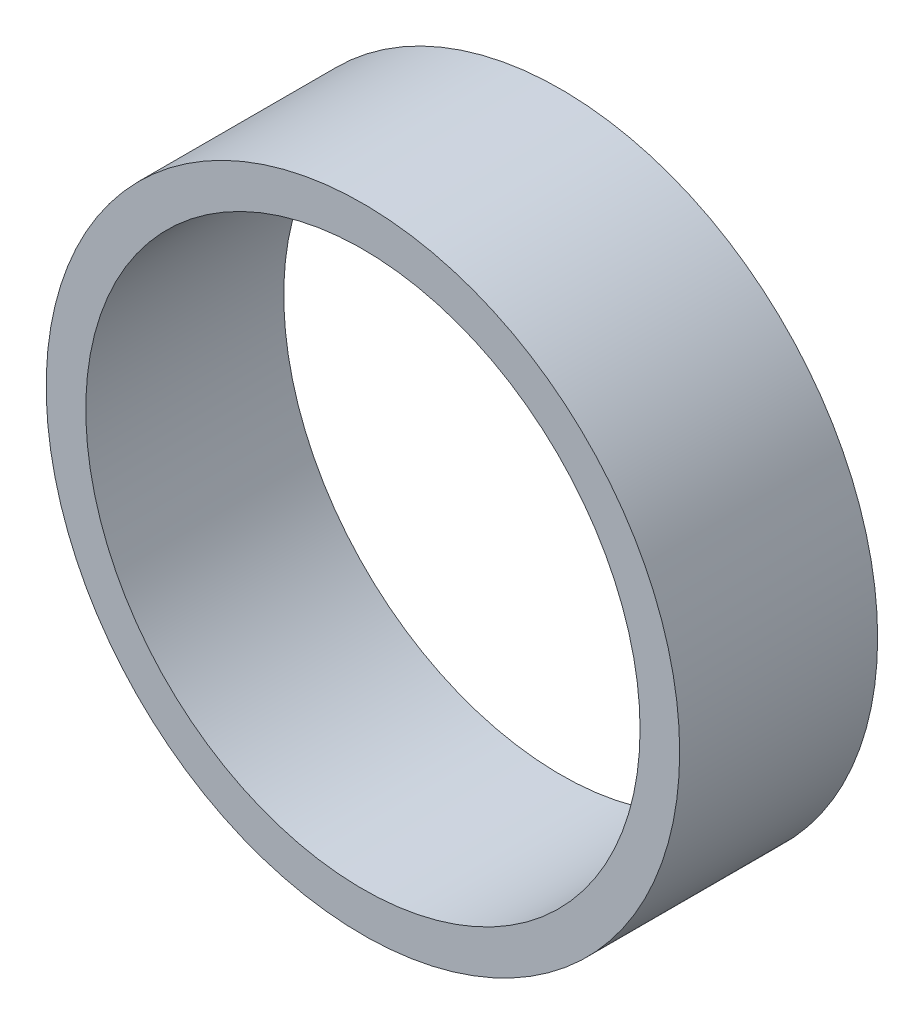
SolidWorks part; units mm, degrees
ref_plane "前视基准面" through (0, 0, 0) normal (0, 0, 1) x (1, 0, 0)
ref_plane "上视基准面" through (0, 0, 0) normal (0, 1, 0) x (1, 0, 0)
ref_plane "右视基准面" through (0, 0, 0) normal (1, 0, 0) x (0, 0, -1)
other "Configuration Table"
sketch "草图1" plane through (0, 0, 0) normal (0, 0, 1) x (1, 0, 0)
  circle A0 centre (0, 0) radius 40
  circle A1 centre (0, 0) radius 35
  point P0 (0, 0)
  dimension "D1" = 70
  dimension "D2" = 80
extrude "凸台-拉伸1" add sketch "草图1" against normal mid plane 25
